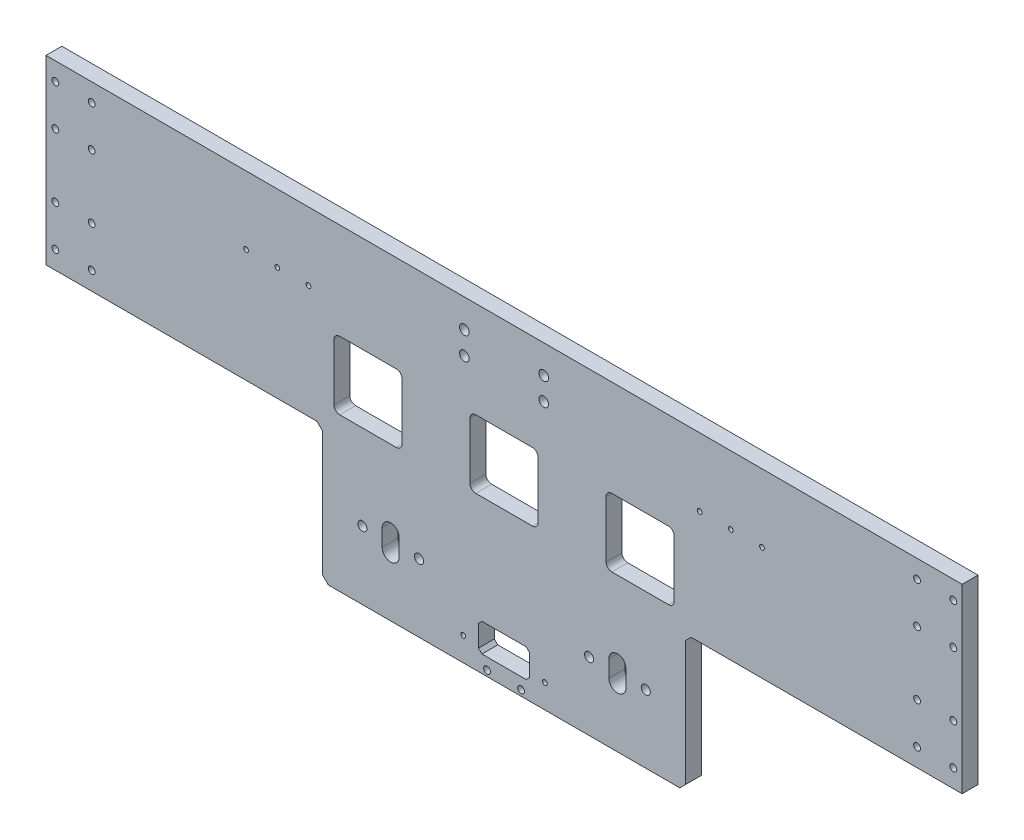
from build123d import *

# Parameters (mm, degrees)
SKETCH1_W                = 808
SKETCH1_H                = 160
BOSS_EXTRUDE1_DEPTH      = 14
F_6_0_6_DIAMETER_HOLE1_D = 6
M10_TAPPED_HOLE2_D       = 8.5
LPATTERN3_COUNT          = 2
LPATTERN3_PITCH          = 92
M5_TAPPED_HOLE1_D        = 4.2
M5_TAPPED_HOLE1_DEPTH    = 16.4
M5_TAPPED_HOLE1_TIP      = 1.2618073
SKETCH7_W                = 320
SKETCH7_H                = 14
BOSS_EXTRUDE2_DEPTH      = 120
SKETCH8_R                = 3
SKETCH8_R_2              = 4
SKETCH8_W                = 45
SKETCH8_H                = 25
CUT_EXTRUDE1_DEPTH       = 824.808230112
CHAMFER1_SIZE            = 3
CHAMFER2_SIZE            = 5
SKETCH10_W               = 60
SKETCH10_H               = 60
CUT_EXTRUDE3_DEPTH       = 824.808230112
FILLET1_R                = 5
M5_TAPPED_HOLE2_D        = 4.2


with BuildPart() as part:
    # Sketch1 → Boss-Extrude1 (new body)
    with BuildSketch(Plane.XY):
        with Locations((404, 80)):
            Rectangle(SKETCH1_W, SKETCH1_H)
    extrude(amount=BOSS_EXTRUDE1_DEPTH)

    # Ø6.0 (6) Diameter Hole1 (through all)
    with Locations(Plane(origin=(8.269330411, 52, 14), x_dir=(1, 0, 0), z_dir=(0, 0, 1))):
        with Locations((0, 0), (32, 0), (0, -36), (32, -36), (760, 0), (792, 0), (792, -36), (760, -36)):
            f_6_0_6_diameter_hole1 = Hole(F_6_0_6_DIAMETER_HOLE1_D / 2)

    # M10 Tapped Hole2 (through all)
    with Locations(Plane(origin=(439, 135, 0), x_dir=(-1, 0, 0), z_dir=(0, 0, -1))):
        with Locations((0, 0), (70, 0), (0, -20), (70, -20)):
            Hole(M10_TAPPED_HOLE2_D / 2)

    # LPattern3: Ø6.0 (6) Diameter Hole1 ×2
    with Locations(*[(0, i * LPATTERN3_PITCH, 0) for i in range(1, LPATTERN3_COUNT)]):
        add(f_6_0_6_diameter_hole1, mode=Mode.SUBTRACT)

    # M5 Tapped Hole1
    with Locations(Plane(origin=(0, 0, 0), x_dir=(-1, 0, 0), z_dir=(0, 0, -1))):
        with Locations((-631.5, 100), (-604, 100), (-576.5, 100), (-231.5, 100), (-204, 100), (-176.5, 100)):
            Hole(M5_TAPPED_HOLE1_D / 2, depth=M5_TAPPED_HOLE1_DEPTH)
            with Locations((0, 0, -(M5_TAPPED_HOLE1_DEPTH + M5_TAPPED_HOLE1_TIP / 2))):  # 118° drill point
                Cone(0, M5_TAPPED_HOLE1_D / 2, M5_TAPPED_HOLE1_TIP, mode=Mode.SUBTRACT)

    # Sketch7 → Boss-Extrude2 (add)
    with BuildSketch(Plane.XZ):
        with Locations((404, 7)):
            Rectangle(SKETCH7_W, SKETCH7_H)
    extrude(amount=BOSS_EXTRUDE2_DEPTH)

    # Sketch8 → Cut-Extrude1 (cut, through all)
    with BuildSketch(Plane(origin=(0, 0, 0), x_dir=(-1, 0, 0), z_dir=(0, 0, -1))):
        with Locations((-419, -115)):
            Circle(SKETCH8_R)
        with Locations(Location((-389, -115, 0), (0, 0, 180))):
            Circle(SKETCH8_R)
        with Locations((-529, -60)):
            Circle(SKETCH8_R_2)
        with Locations((-479, -60)):
            Circle(SKETCH8_R_2)
        with Locations(Location((-329, -60, 0), (0, 0, 180))):
            Circle(SKETCH8_R_2)
        with Locations(Location((-279, -60, 0), (0, 0, 180))):
            Circle(SKETCH8_R_2)
        with Locations((-404, -92.5)):
            Rectangle(SKETCH8_W, SKETCH8_H)
        with BuildLine():
            Line((-496.5, -52.5), (-496.5, -67.5))
            ThreePointArc((-496.5, -67.5), (-504, -75), (-511.5, -67.5))
            Line((-511.5, -67.5), (-511.5, -52.5))
            ThreePointArc((-511.5, -52.5), (-504, -45), (-496.5, -52.5))
        make_face()
        with BuildLine():
            Line((-311.5, -52.5), (-311.5, -67.5))
            ThreePointArc((-311.5, -67.5), (-304, -75), (-296.5, -67.5))
            Line((-296.5, -67.5), (-296.5, -52.5))
            ThreePointArc((-296.5, -52.5), (-304, -45), (-311.5, -52.5))
        make_face()
    extrude(amount=-CUT_EXTRUDE1_DEPTH, mode=Mode.SUBTRACT)

    # Chamfer1
    chamfer1_edges = [part.edges().sort_by_distance(p)[0] for p in [
        (426.5, -105, 7),
        (426.5, -80, 7),
        (381.5, -80, 7),
        (381.5, -105, 7),
    ]]
    chamfer(chamfer1_edges, length=CHAMFER1_SIZE)

    # Chamfer2
    chamfer2_edges = [part.edges().sort_by_distance(p)[0] for p in [
        (244, 0, 7),
        (564, 0, 7),
        (244, -120, 7),
        (564, -120, 7),
    ]]
    chamfer(chamfer2_edges, length=CHAMFER2_SIZE)

    # Sketch10 → Cut-Extrude3 (cut, through all)
    with BuildSketch(Plane(origin=(0, 0, 0), x_dir=(-1, 0, 0), z_dir=(0, 0, -1))):
        with Locations((-524, 45)):
            Rectangle(SKETCH10_W, SKETCH10_H)
        with Locations((-404, 45)):
            Rectangle(SKETCH10_W, SKETCH10_H)
        with Locations((-284, 45)):
            Rectangle(SKETCH10_W, SKETCH10_H)
    extrude(amount=-CUT_EXTRUDE3_DEPTH, mode=Mode.SUBTRACT)

    # Fillet1
    fillet1_edges = [part.edges().sort_by_distance(p)[0] for p in [
        (554, 15, 7),
        (554, 75, 7),
        (494, 75, 7),
        (494, 15, 7),
        (434, 15, 7),
        (434, 75, 7),
        (374, 75, 7),
        (374, 15, 7),
        (314, 15, 7),
        (314, 75, 7),
        (254, 75, 7),
        (254, 15, 7),
    ]]
    fillet(fillet1_edges, radius=FILLET1_R)

    # M5 Tapped Hole2 (through all)
    with Locations(Plane.XY.offset(14)):
        with Locations((368, -99), (440, -99)):
            Hole(M5_TAPPED_HOLE2_D / 2)


solid = part.part
